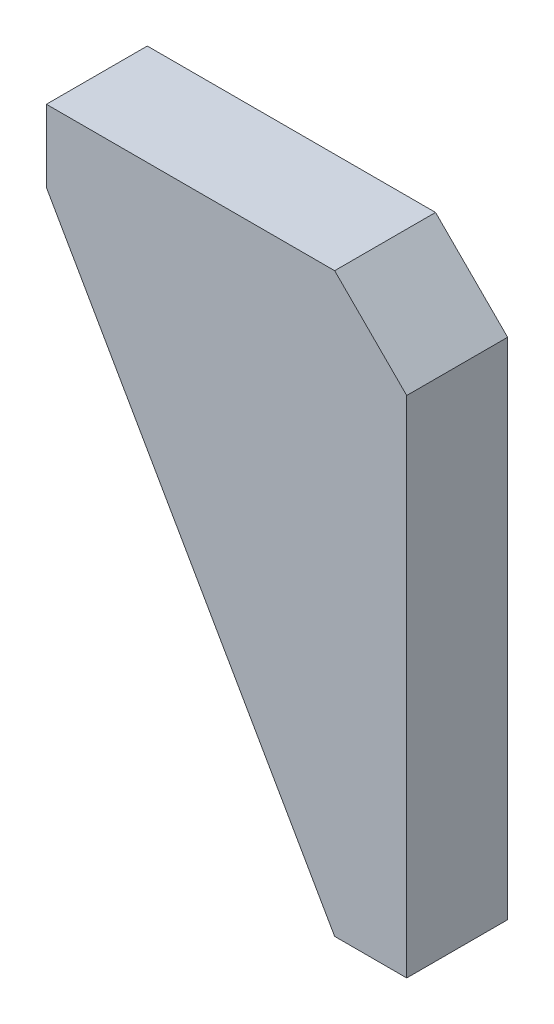
SolidWorks part; units mm, degrees
material "Q235"
ref_plane "Front Plane" through (0, 0, 0) normal (0, 0, 1) x (1, 0, 0)
ref_plane "Top Plane" through (0, 0, 0) normal (0, 1, 0) x (1, 0, 0)
ref_plane "Right Plane" through (0, 0, 0) normal (1, 0, 0) x (0, 0, -1)
sketch "Sketch1" plane through (0, 0, 0) normal (0, 0, -1) x (1, 0, 0)
  line L0 (0, 0) -> (0, 80)
  line L1 (0, 80) -> (-10, 80)
  line L2 (-10, 80) -> (-50, 10)
  line L3 (-50, 10) -> (-50, 0)
  line L4 (-50, 0) -> (0, 0)
  dimension "D3" = 10
  dimension "D4" = 10
  dimension "D1" = 50
  dimension "D2" = 80
extrude "Boss-Extrude1" add sketch "Sketch1" along normal blind 14
chamfer "Chamfer1" distance 10 angle 45 1 edges at (0, 0, -7)
